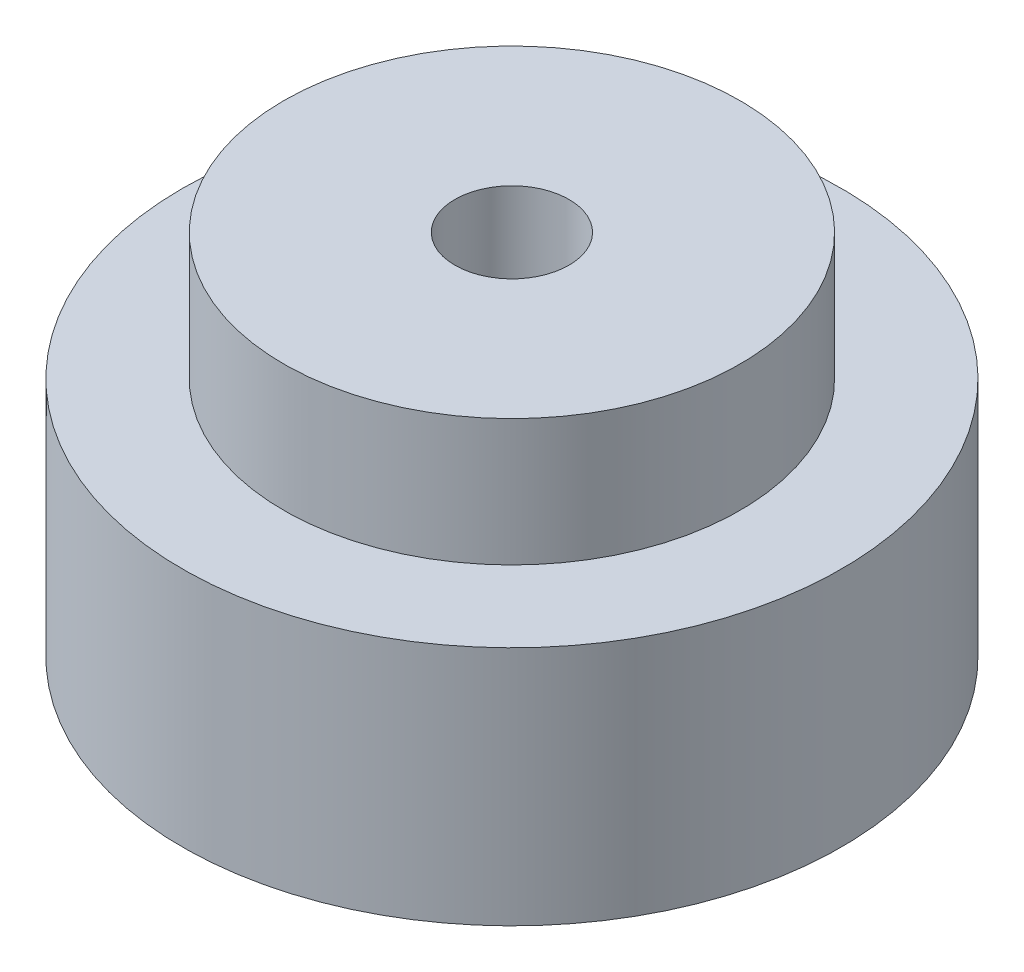
from build123d import *

# Parameters (mm, degrees)
M10X1_0_TAPPED_HOLE1_D = 9
SKETCH4_R              = 3
CUT_EXTRUDE1_DEPTH     = 47.829477896


with BuildPart() as part:
    # Sketch1 → Revolve1 (revolve)
    with BuildSketch(Plane.XY, mode=Mode.PRIVATE) as revolve1_sk:
        Polygon((20, 0), (26, 0), (26, 19), (18, 19), (18, 29), (0, 29), (0, 17), (5, 17), (20, 11), align=None)
    revolve(revolve1_sk.sketch.rotate(Axis((0, 29.712230849, 0), (0, -1, 0)), 180), axis=Axis((0, 29.712230849, 0), (0, -1, 0)))

    # M10x1.0 Tapped Hole1 (through all)
    with Locations(Plane(origin=(0, 29, 0), x_dir=(1, 0, 0), z_dir=(0, 1, 0))):
        with Locations((0, 0)):
            Hole(M10X1_0_TAPPED_HOLE1_D / 2)

    # Sketch4 → Cut-Extrude1 (cut, through all)
    with BuildSketch(Plane(origin=(0, 0, 0), x_dir=(0, 0, -1), z_dir=(1, 0, 0))):
        with Locations(Location((0, 9, 0), (0, 0, 270.000000001))):
            Circle(SKETCH4_R)
    extrude(amount=-CUT_EXTRUDE1_DEPTH, mode=Mode.SUBTRACT)


solid = part.part
